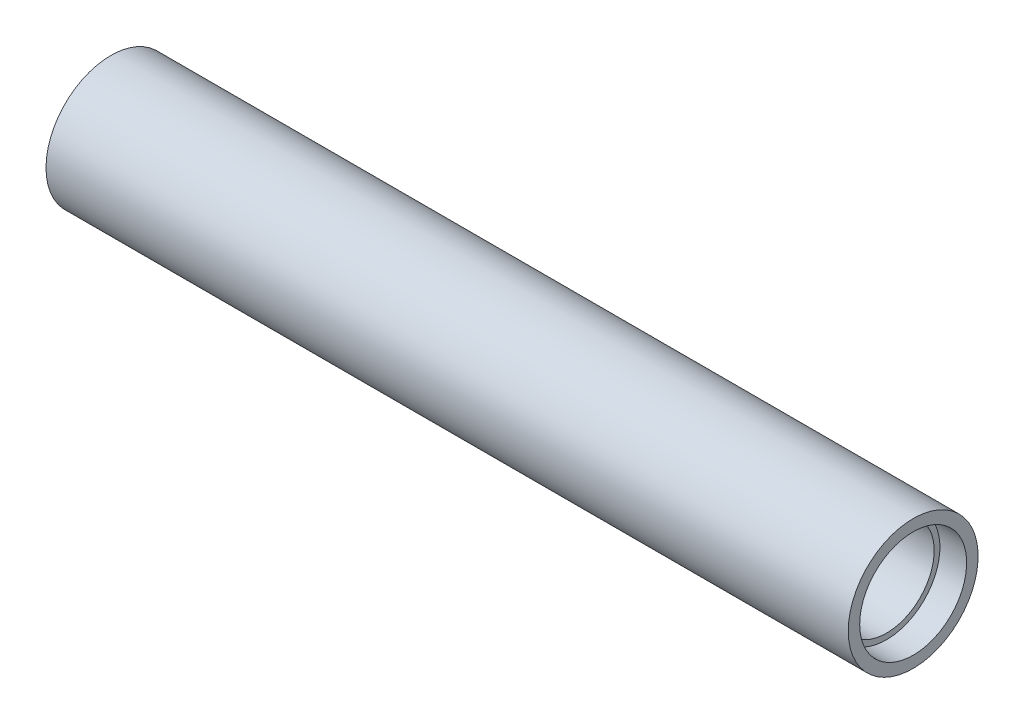
SolidWorks part; units mm, degrees
ref_plane "前视基准面" through (0, 0, 0) normal (0, 0, 1) x (1, 0, 0)
ref_plane "上视基准面" through (0, 0, 0) normal (0, 1, 0) x (1, 0, 0)
ref_plane "右视基准面" through (0, 0, 0) normal (1, 0, 0) x (0, 0, -1)
sketch "草图1" plane through (0, 0, 0) normal (0, 0, 1) x (1, 0, 0)
  line L0 (0, 0) -> (0, 17) construction
  line L1 (105, 17) -> (-105, 17)
  line L2 (-105, 17) -> (-105, 14)
  line L3 (-105, 14) -> (-98, 14)
  line L4 (-98, 14) -> (-98, 12.5)
  line L5 (-98, 12.5) -> (98, 12.5)
  line L6 (98, 14) -> (98, 12.5)
  line L7 (105, 14) -> (98, 14)
  line L8 (105, 17) -> (105, 14)
  line L9 (0, 0) -> (46.6922, 0) construction
  point P9 (0, 12.5)
  dimension "D1" = 1.5
  dimension "D2" = 3
  dimension "D3" = 105
  dimension "D4" = 7
  dimension "D5" = 14
revolve "旋转1" add sketch "草图1" angle 360 about L9
